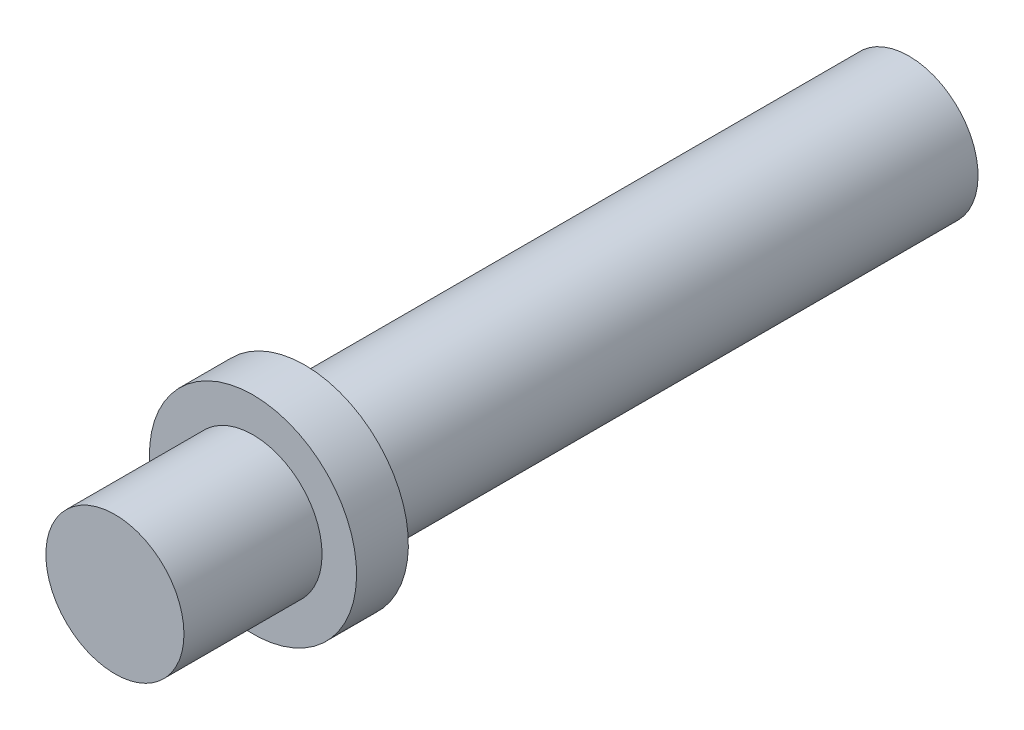
SolidWorks part; units mm, degrees
ref_plane "前视基准面" through (0, 0, 0) normal (0, 0, 1) x (1, 0, 0)
ref_plane "上视基准面" through (0, 0, 0) normal (0, 1, 0) x (1, 0, 0)
ref_plane "右视基准面" through (0, 0, 0) normal (1, 0, 0) x (0, 0, -1)
sketch "草图1" plane through (0, 0, 0) normal (0, 0, 1) x (1, 0, 0)
  circle A0 centre (-145.5047, 180.5689) radius 4 construction
  circle A1 centre (-145.5047, 180.5689) radius 4
extrude "凸台-拉伸1" add sketch "草图1" against normal up to surface (8 mm away)
sketch "草图2" plane through (0, 0, -8) normal (0, 0, -1) x (-1, 0, 0)
  circle A0 centre (145.5047, 180.5689) radius 6
  dimension "D1" = 12
extrude "凸台-拉伸2" add sketch "草图2" along normal blind 3
sketch "草图3" plane through (0, 0, -11) normal (0, 0, -1) x (-1, 0, 0)
  circle A0 centre (145.5047, 180.5689) radius 4 construction
  circle A1 centre (145.5047, 180.5689) radius 4
extrude "凸台-拉伸3" add sketch "草图3" along normal blind 30
sketch "草图4" plane through (0, 0, -41) normal (0, 0, -1) x (-1, 0, 0)
  circle A1 centre (145.5047, 180.5689) radius 4
  circle A2 centre (145.5047, 180.5689) radius 4
  dimension "D1" = 0
extrude "凸台-拉伸4" add sketch "草图4" along normal blind 5
